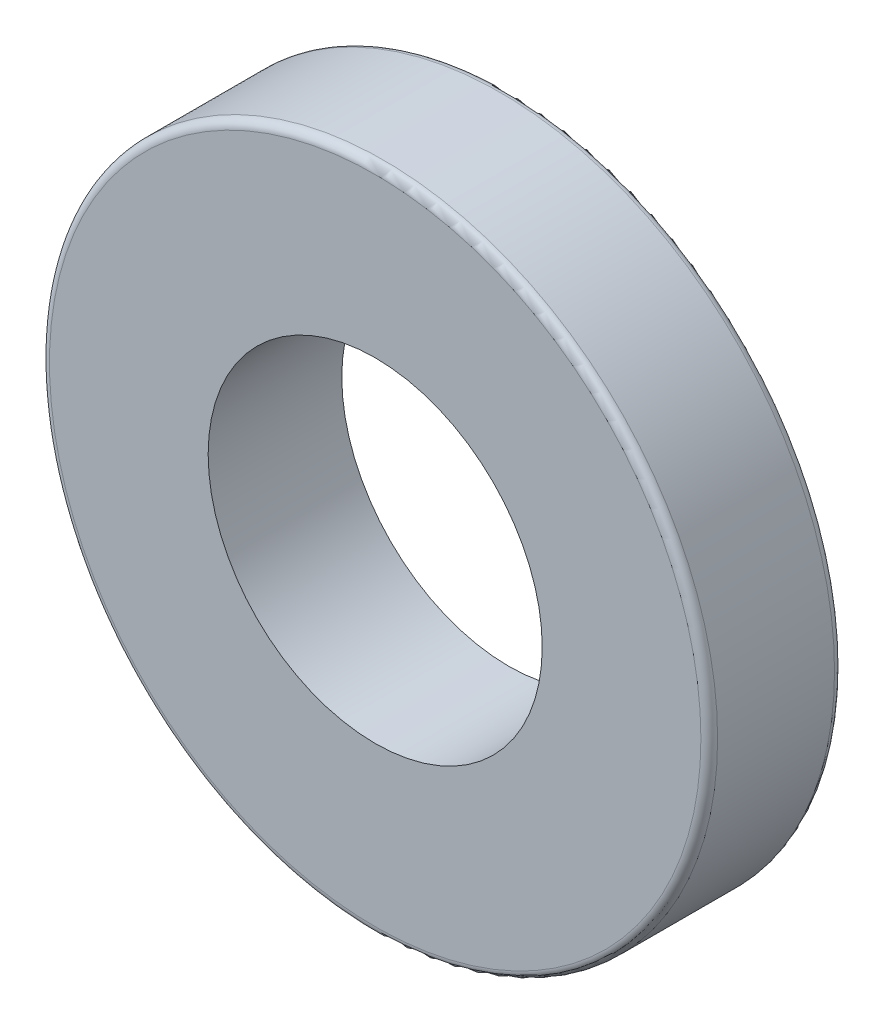
SolidWorks part; units mm, degrees
material "标准件"
ref_plane "前视基准面" through (0, 0, 0) normal (0, 0, 1) x (1, 0, 0)
ref_plane "上视基准面" through (0, 0, 0) normal (0, 1, 0) x (1, 0, 0)
ref_plane "右视基准面" through (0, 0, 0) normal (1, 0, 0) x (0, 0, -1)
sketch "草图1" plane through (0, 0, 0) normal (0, 0, 1) x (1, 0, 0)
  circle A0 centre (0, 0) radius 10
  circle A1 centre (0, 0) radius 20
  dimension "D1" = 20
  dimension "D2" = 40
extrude "凸台-拉伸1" add sketch "草图1" along normal mid plane 8
fillet "圆角1" radius 0.5 2 edges at (20, 0, -4) (20, 0, 4)
